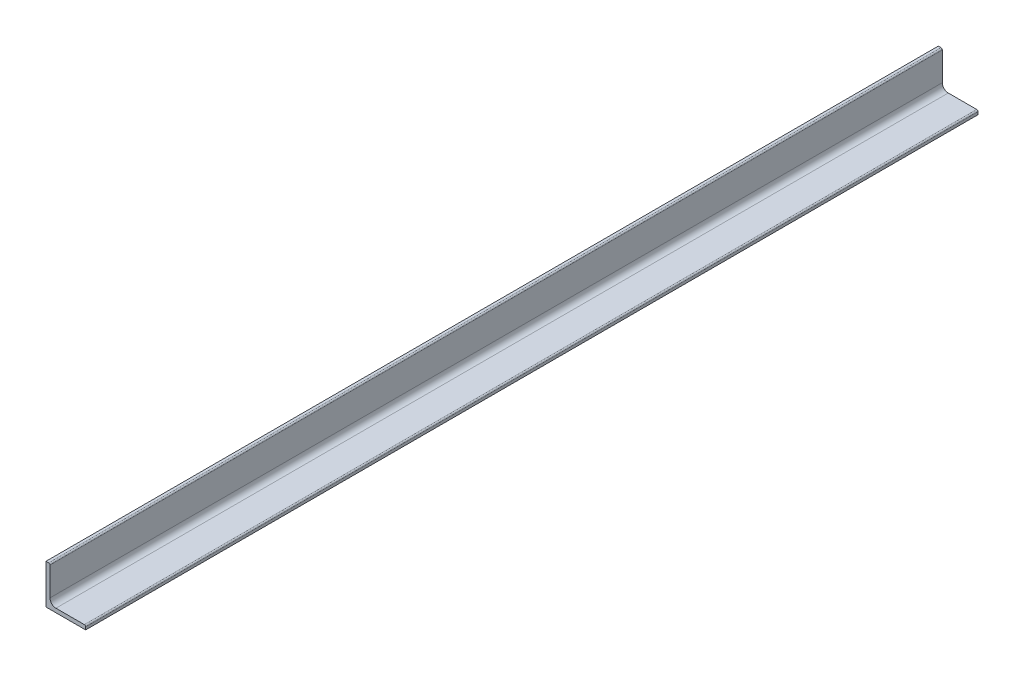
SolidWorks part; units mm, degrees
material "Plain Carbon Steel"
ref_plane "Plane1" through (0, 0, 0) normal (0, 0, 1) x (1, 0, 0)
ref_plane "Plane2" through (0, 0, 0) normal (0, 1, 0) x (1, 0, 0)
ref_plane "Plane3" through (0, 0, 0) normal (1, 0, 0) x (0, 0, -1)
sketch "Sketch1" plane through (0, 0, 0) normal (0, 0, 1) x (1, 0, 0)
  line L0 (0, 0) -> (0, 30)
  line L1 (0, 15) -> (3, 15) construction
  line L2 (3, 29) -> (3, 7.5)
  line L3 (7.5, 3) -> (29, 3)
  line L4 (15, 3) -> (15, 0) construction
  line L5 (30, 0) -> (0, 0)
  line L6 (0, 30) -> (2, 30)
  line L7 (30, 0) -> (30, 2)
  arc A0 (30, 2) -> (29, 3) centre (29, 2) ccw
  arc A1 (2, 30) -> (3, 29) centre (2, 29) cw
  arc A2 (7.5, 3) -> (3, 7.5) centre (7.5, 7.5) cw
  point P10 (15, 0)
  point P14 (0, 15)
  point P15 (3, 15)
  point P16 (15, 3)
  point P17 (3, 30)
  point P18 (30, 3)
  point P21 (30, 3)
  point P24 (3, 30)
extrude "Boss-Extrude1" add sketch "Sketch1" along normal mid plane 675 contours L2 A2 L3 A0 L7 L5 L0 L6 A1
equation "\"D2@Sketch1\" = \"D1@Sketch1\" / 3"
